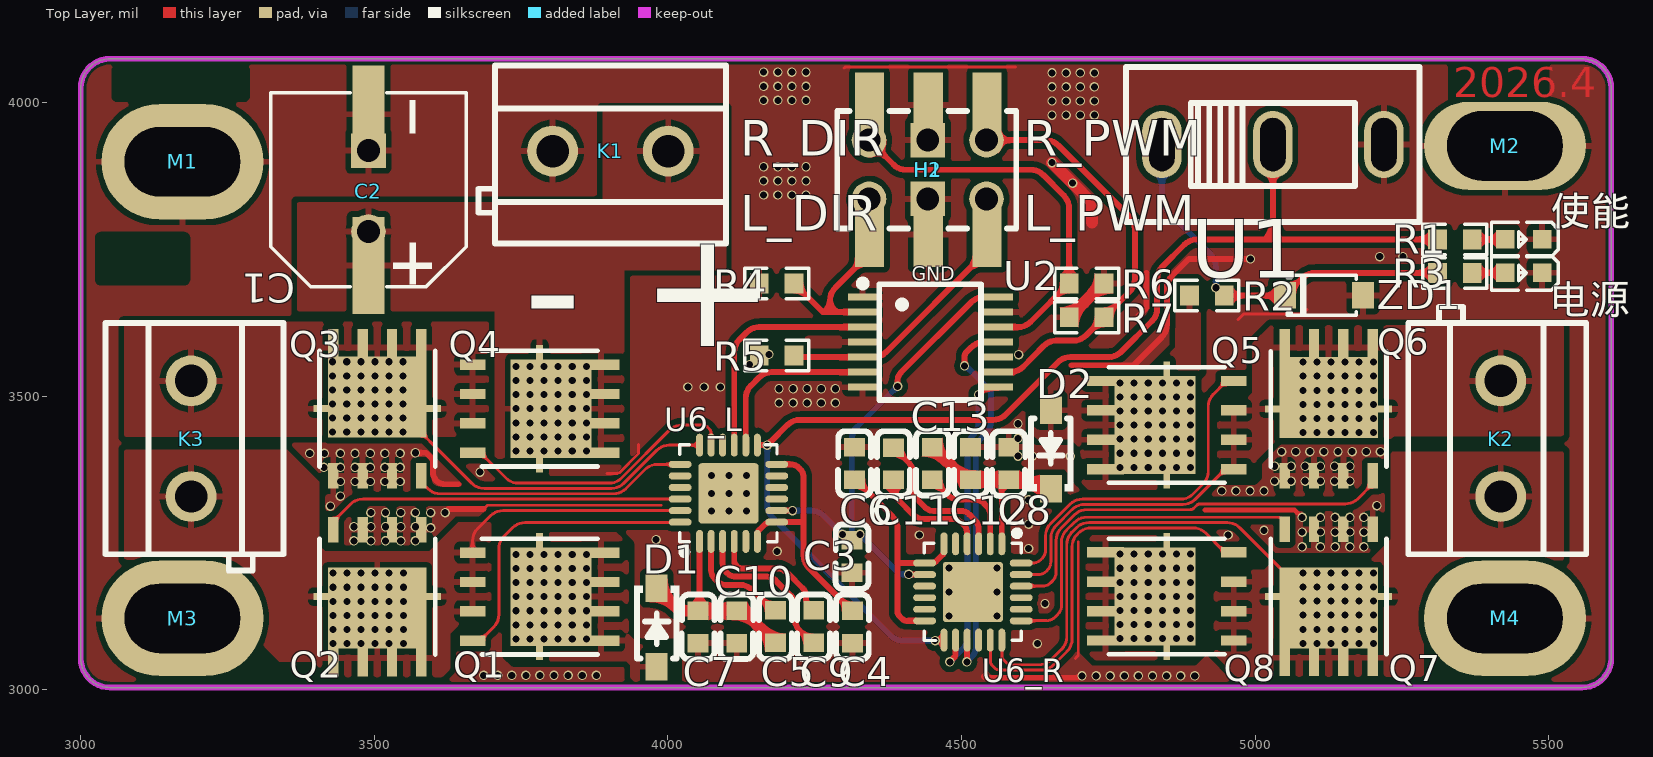
[diagram p0: Top Layer view]
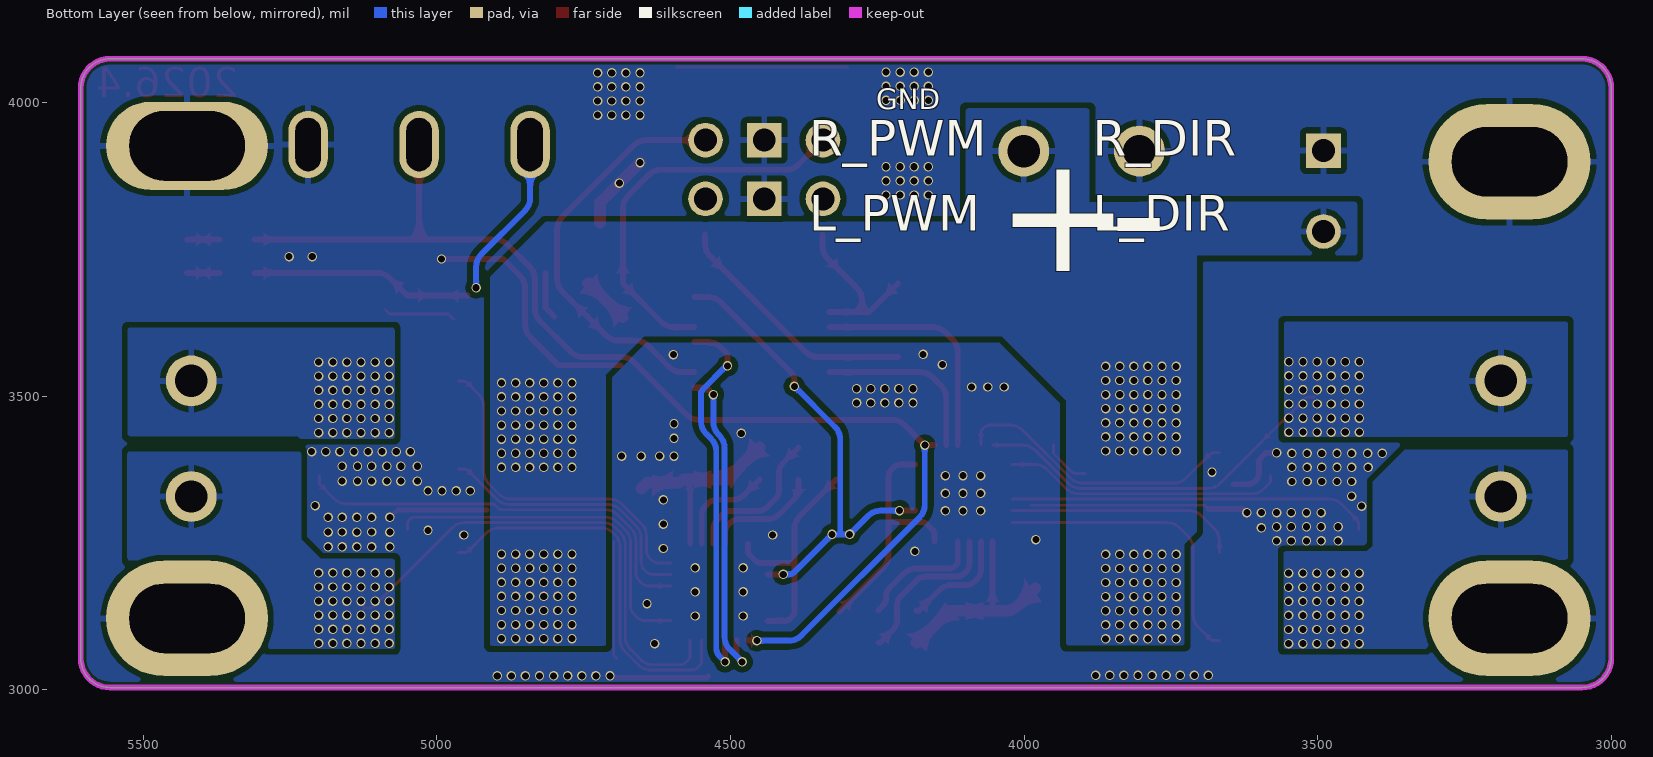
[diagram p1: Bottom Layer view, seen from below]
# Altium PCB MISC62357.pcbdoc (part 1 of 2)
Units mil, origin at the board's own origin, x right, y up, seen from the top; angles counter-clockwise.
Board outline 2606.3 x 1070.87 mil, 2 copper layers (Top Layer, Bottom Layer), stack 62.206 mil thick; 46 components, 37 nets, 219 pads, 514 vias.

## Layer stack, top to bottom
Top Solder Mask Layer: solder mask 0.394, Dk 3.3
Top Layer: signal copper 1.379
Dielectric1: surface 59.449, FR4, Dk 4.5
Bottom Layer: signal copper 1.378
Bottom Solder Mask Layer: solder mask 0.394, Dk 3.3

## Board outline
3050,4074.6 ccw(c3050,4024.6) 3000,4024.6 3000,3053.73 ccw(c3050,3053.73) 3050,3003.73 5556.3,3003.73 ccw(c5556.3,3053.73) 5606.3,3053.73 5606.3,4024.6 ccw(c5556.3,4024.6) 5556.3,4074.6

## Design rules (kind name [scope] priority, off if disabled: settings)
BoardOutlineClearance copperThickness2oz_1 [All] p2 off: genericclearance=8 ignorepadtopadclearanceinfootprint=FALSE except(0: Arc-SplitContinuation Track-SplitContinuation SMDPad-SplitContinuation THPad-SplitContinuation Via-SplitContinuation Fill-SplitContinuation Region-SplitContinuation Poly-SplitContinuation Text-SplitContinuation Hole-SplitContinuation; 6: Arc-CutoutEdge Track-CutoutEdge SMDPad-CutoutEdge THPad-CutoutEdge Via-CutoutEdge Text-CutoutEdge; 6.9: Hole-OutlineEdge Hole-CutoutEdge; 10: Poly-OutlineEdge Poly-CutoutEdge; 11.8: Arc-OutlineEdge Track-OutlineEdge SMDPad-OutlineEdge THPad-OutlineEdge Via-OutlineEdge Fill-OutlineEdge Region-OutlineEdge Text-OutlineEdge Fill-CutoutEdge Region-CutoutEdge)
BoardOutlineClearance Plane_innerPlane_1 [All] p4 off: genericclearance=4 ignorepadtopadclearanceinfootprint=FALSE except(0: Arc-SplitContinuation Track-SplitContinuation SMDPad-SplitContinuation THPad-SplitContinuation Via-SplitContinuation Fill-SplitContinuation Region-SplitContinuation Poly-SplitContinuation Text-SplitContinuation Hole-SplitContinuation; 6: Arc-CutoutEdge Track-CutoutEdge SMDPad-CutoutEdge THPad-CutoutEdge Via-CutoutEdge Text-CutoutEdge; 6.9: Hole-OutlineEdge Hole-CutoutEdge; 10: Poly-OutlineEdge Poly-CutoutEdge; 11.8: Arc-OutlineEdge Track-OutlineEdge SMDPad-OutlineEdge THPad-OutlineEdge Via-OutlineEdge Fill-OutlineEdge Region-OutlineEdge Text-OutlineEdge Fill-CutoutEdge Region-CutoutEdge)
BoardOutlineClearance Copper_copperRegion_1 [All] p6 off: genericclearance=4 ignorepadtopadclearanceinfootprint=FALSE except(0: Arc-SplitContinuation Track-SplitContinuation SMDPad-SplitContinuation THPad-SplitContinuation Via-SplitContinuation Fill-SplitContinuation Region-SplitContinuation Poly-SplitContinuation Text-SplitContinuation Hole-SplitContinuation; 6: Arc-CutoutEdge Track-CutoutEdge SMDPad-CutoutEdge THPad-CutoutEdge Via-CutoutEdge Text-CutoutEdge; 6.9: Hole-OutlineEdge Hole-CutoutEdge; 10: Poly-OutlineEdge Poly-CutoutEdge; 11.8: Arc-OutlineEdge Track-OutlineEdge SMDPad-OutlineEdge THPad-OutlineEdge Via-OutlineEdge Fill-OutlineEdge Region-OutlineEdge Text-OutlineEdge Fill-CutoutEdge Region-CutoutEdge)
BoardOutlineClearance Copper_直连_1 [All] p8 off: genericclearance=4 ignorepadtopadclearanceinfootprint=FALSE except(0: Arc-SplitContinuation Track-SplitContinuation SMDPad-SplitContinuation THPad-SplitContinuation Via-SplitContinuation Fill-SplitContinuation Region-SplitContinuation Poly-SplitContinuation Text-SplitContinuation Hole-SplitContinuation; 6: Arc-CutoutEdge Track-CutoutEdge SMDPad-CutoutEdge THPad-CutoutEdge Via-CutoutEdge Text-CutoutEdge; 6.9: Hole-OutlineEdge Hole-CutoutEdge; 10: Poly-OutlineEdge Poly-CutoutEdge; 11.8: Arc-OutlineEdge Track-OutlineEdge SMDPad-OutlineEdge THPad-OutlineEdge Via-OutlineEdge Fill-OutlineEdge Region-OutlineEdge Text-OutlineEdge Fill-CutoutEdge Region-CutoutEdge)
BoardOutlineClearance Copper_18_1 [All] p10 off: genericclearance=4 ignorepadtopadclearanceinfootprint=FALSE except(0: Arc-SplitContinuation Track-SplitContinuation SMDPad-SplitContinuation THPad-SplitContinuation Via-SplitContinuation Fill-SplitContinuation Region-SplitContinuation Poly-SplitContinuation Text-SplitContinuation Hole-SplitContinuation; 6: Arc-CutoutEdge Track-CutoutEdge SMDPad-CutoutEdge THPad-CutoutEdge Via-CutoutEdge Text-CutoutEdge; 6.9: Hole-OutlineEdge Hole-CutoutEdge; 10: Poly-OutlineEdge Poly-CutoutEdge; 11.8: Arc-OutlineEdge Track-OutlineEdge SMDPad-OutlineEdge THPad-OutlineEdge Via-OutlineEdge Fill-OutlineEdge Region-OutlineEdge Text-OutlineEdge Fill-CutoutEdge Region-CutoutEdge)
BoardOutlineClearance Copper_18_copperThickness1oz_1 [All] p12 off: genericclearance=4 ignorepadtopadclearanceinfootprint=FALSE except(0: Arc-SplitContinuation Track-SplitContinuation SMDPad-SplitContinuation THPad-SplitContinuation Via-SplitContinuation Fill-SplitContinuation Region-SplitContinuation Poly-SplitContinuation Text-SplitContinuation Hole-SplitContinuation; 6: Arc-CutoutEdge Track-CutoutEdge SMDPad-CutoutEdge THPad-CutoutEdge Via-CutoutEdge Text-CutoutEdge; 6.9: Hole-OutlineEdge Hole-CutoutEdge; 10: Poly-OutlineEdge Poly-CutoutEdge; 11.8: Arc-OutlineEdge Track-OutlineEdge SMDPad-OutlineEdge THPad-OutlineEdge Via-OutlineEdge Fill-OutlineEdge Region-OutlineEdge Text-OutlineEdge Fill-CutoutEdge Region-CutoutEdge)
BoardOutlineClearance Copper_18_Copper_copperRegion_1 [All] p14 off: genericclearance=4 ignorepadtopadclearanceinfootprint=FALSE except(0: Arc-SplitContinuation Track-SplitContinuation SMDPad-SplitContinuation THPad-SplitContinuation Via-SplitContinuation Fill-SplitContinuation Region-SplitContinuation Poly-SplitContinuation Text-SplitContinuation Hole-SplitContinuation; 6: Arc-CutoutEdge Track-CutoutEdge SMDPad-CutoutEdge THPad-CutoutEdge Via-CutoutEdge Text-CutoutEdge; 6.9: Hole-OutlineEdge Hole-CutoutEdge; 10: Poly-OutlineEdge Poly-CutoutEdge; 11.8: Arc-OutlineEdge Track-OutlineEdge SMDPad-OutlineEdge THPad-OutlineEdge Via-OutlineEdge Fill-OutlineEdge Region-OutlineEdge Text-OutlineEdge Fill-CutoutEdge Region-CutoutEdge)
BoardOutlineClearance Copper_copperRegion_Copper_18_1 [All] p16 off: genericclearance=4 ignorepadtopadclearanceinfootprint=FALSE except(0: Arc-SplitContinuation Track-SplitContinuation SMDPad-SplitContinuation THPad-SplitContinuation Via-SplitContinuation Fill-SplitContinuation Region-SplitContinuation Poly-SplitContinuation Text-SplitContinuation Hole-SplitContinuation; 6: Arc-CutoutEdge Track-CutoutEdge SMDPad-CutoutEdge THPad-CutoutEdge Via-CutoutEdge Text-CutoutEdge; 6.9: Hole-OutlineEdge Hole-CutoutEdge; 10: Poly-OutlineEdge Poly-CutoutEdge; 11.8: Arc-OutlineEdge Track-OutlineEdge SMDPad-OutlineEdge THPad-OutlineEdge Via-OutlineEdge Fill-OutlineEdge Region-OutlineEdge Text-OutlineEdge Fill-CutoutEdge Region-CutoutEdge)
BoardOutlineClearance Copper_copperRegion_Copper_copperRegion_1 [All] p18 off: genericclearance=4 ignorepadtopadclearanceinfootprint=FALSE except(0: Arc-SplitContinuation Track-SplitContinuation SMDPad-SplitContinuation THPad-SplitContinuation Via-SplitContinuation Fill-SplitContinuation Region-SplitContinuation Poly-SplitContinuation Text-SplitContinuation Hole-SplitContinuation; 6: Arc-CutoutEdge Track-CutoutEdge SMDPad-CutoutEdge THPad-CutoutEdge Via-CutoutEdge Text-CutoutEdge; 6.9: Hole-OutlineEdge Hole-CutoutEdge; 10: Poly-OutlineEdge Poly-CutoutEdge; 11.8: Arc-OutlineEdge Track-OutlineEdge SMDPad-OutlineEdge THPad-OutlineEdge Via-OutlineEdge Fill-OutlineEdge Region-OutlineEdge Text-OutlineEdge Fill-CutoutEdge Region-CutoutEdge)
BoardOutlineClearance copperThickness1oz_1 [All] p20: genericclearance=4 ignorepadtopadclearanceinfootprint=FALSE except(0: Arc-SplitContinuation Track-SplitContinuation SMDPad-SplitContinuation THPad-SplitContinuation Via-SplitContinuation Fill-SplitContinuation Region-SplitContinuation Poly-SplitContinuation Text-SplitContinuation Hole-SplitContinuation; 6: Arc-CutoutEdge Track-CutoutEdge SMDPad-CutoutEdge THPad-CutoutEdge Via-CutoutEdge Text-CutoutEdge; 6.9: Hole-OutlineEdge Hole-CutoutEdge; 10: Poly-OutlineEdge Poly-CutoutEdge; 11.8: Arc-OutlineEdge Track-OutlineEdge SMDPad-OutlineEdge THPad-OutlineEdge Via-OutlineEdge Fill-OutlineEdge Region-OutlineEdge Text-OutlineEdge Fill-CutoutEdge Region-CutoutEdge)
Clearance copperThickness2oz [All] p1 off: gap=8 ignorepadtopadclearanceinfootprint=FALSE except(6: SMDPad-Track SMDPad-SMDPad THPad-Track SMDPad-THPad THPad-THPad Track-Via SMDPad-Via THPad-Via Via-Via Fill-SMDPad Region-SMDPad Fill-THPad Region-THPad Fill-Via Region-Via Arc-Track Arc-SMDPad Arc-THPad Arc-Via Fill-Arc Region-Arc Arc-Arc Text-Track SMDPad-Text Text-THPad Text-Via Fill-Text Region-Text Arc-Text Text-Text; 6.9: Hole-Track Hole-SMDPad Hole-THPad Hole-Via Fill-Hole Region-Hole Hole-Arc Hole-Text; 10: Poly-Track Poly-SMDPad Poly-THPad Poly-Via Poly-Fill Poly-Region Poly-Poly Poly-Arc Poly-Text Poly-Hole; 11.8: Fill-Track Region-Track; 20: Fill-Fill Fill-Region Region-Region)
Clearance Plane_innerPlane [All] p3 off: gap=4 ignorepadtopadclearanceinfootprint=FALSE except(6: SMDPad-Track SMDPad-SMDPad THPad-Track SMDPad-THPad THPad-THPad Track-Via SMDPad-Via THPad-Via Via-Via Fill-SMDPad Region-SMDPad Fill-THPad Region-THPad Fill-Via Region-Via Arc-Track Arc-SMDPad Arc-THPad Arc-Via Fill-Arc Region-Arc Arc-Arc Text-Track SMDPad-Text Text-THPad Text-Via Fill-Text Region-Text Arc-Text Text-Text; 6.9: Hole-Track Hole-SMDPad Hole-THPad Hole-Via Fill-Hole Region-Hole Hole-Arc Hole-Text; 10: Poly-Track Poly-SMDPad Poly-THPad Poly-Via Poly-Fill Poly-Region Poly-Poly Poly-Arc Poly-Text Poly-Hole; 11.8: Fill-Track Region-Track; 12: Fill-Fill Fill-Region Region-Region)
Clearance Copper_copperRegion [All] p5 off: gap=4 ignorepadtopadclearanceinfootprint=FALSE except(6: SMDPad-Track SMDPad-SMDPad THPad-Track SMDPad-THPad THPad-THPad Track-Via SMDPad-Via THPad-Via Via-Via Fill-SMDPad Region-SMDPad Fill-THPad Region-THPad Fill-Via Region-Via Arc-Track Arc-SMDPad Arc-THPad Arc-Via Fill-Arc Region-Arc Arc-Arc Text-Track SMDPad-Text Text-THPad Text-Via Fill-Text Region-Text Arc-Text Text-Text; 6.9: Hole-Track Hole-SMDPad Hole-THPad Hole-Via Fill-Hole Region-Hole Hole-Arc Hole-Text; 10: Poly-Track Poly-SMDPad Poly-THPad Poly-Via Poly-Fill Poly-Region Poly-Poly Poly-Arc Poly-Text Poly-Hole; 11.8: Fill-Track Region-Track; 12: Fill-Fill Fill-Region Region-Region)
Clearance Copper_直连 [All] p7 off: gap=4 ignorepadtopadclearanceinfootprint=FALSE except(6: SMDPad-Track SMDPad-SMDPad THPad-Track SMDPad-THPad THPad-THPad Track-Via SMDPad-Via THPad-Via Via-Via Fill-SMDPad Region-SMDPad Fill-THPad Region-THPad Fill-Via Region-Via Arc-Track Arc-SMDPad Arc-THPad Arc-Via Fill-Arc Region-Arc Arc-Arc Text-Track SMDPad-Text Text-THPad Text-Via Fill-Text Region-Text Arc-Text Text-Text; 6.9: Hole-Track Hole-SMDPad Hole-THPad Hole-Via Fill-Hole Region-Hole Hole-Arc Hole-Text; 10: Poly-Track Poly-SMDPad Poly-THPad Poly-Via Poly-Fill Poly-Region Poly-Poly Poly-Arc Poly-Text Poly-Hole; 11.8: Fill-Track Region-Track; 12: Fill-Fill Fill-Region Region-Region)
Clearance Copper_18 [All] p9 off: gap=4 ignorepadtopadclearanceinfootprint=FALSE except(6: SMDPad-Track SMDPad-SMDPad THPad-Track SMDPad-THPad THPad-THPad Track-Via SMDPad-Via THPad-Via Via-Via Fill-SMDPad Region-SMDPad Fill-THPad Region-THPad Fill-Via Region-Via Arc-Track Arc-SMDPad Arc-THPad Arc-Via Fill-Arc Region-Arc Arc-Arc Text-Track SMDPad-Text Text-THPad Text-Via Fill-Text Region-Text Arc-Text Text-Text; 6.9: Hole-Track Hole-SMDPad Hole-THPad Hole-Via Fill-Hole Region-Hole Hole-Arc Hole-Text; 10: Poly-Track Poly-SMDPad Poly-THPad Poly-Via Poly-Fill Poly-Region Poly-Poly Poly-Arc Poly-Text Poly-Hole; 11.8: Fill-Track Region-Track; 12: Fill-Fill Fill-Region Region-Region)
Clearance Copper_18_copperThickness1oz [All] p11 off: gap=4 ignorepadtopadclearanceinfootprint=FALSE except(6: SMDPad-Track SMDPad-SMDPad THPad-Track SMDPad-THPad THPad-THPad Track-Via SMDPad-Via THPad-Via Via-Via Fill-SMDPad Region-SMDPad Fill-THPad Region-THPad Fill-Via Region-Via Arc-Track Arc-SMDPad Arc-THPad Arc-Via Fill-Arc Region-Arc Arc-Arc Text-Track SMDPad-Text Text-THPad Text-Via Fill-Text Region-Text Arc-Text Text-Text; 6.9: Hole-Track Hole-SMDPad Hole-THPad Hole-Via Fill-Hole Region-Hole Hole-Arc Hole-Text; 10: Poly-Track Poly-SMDPad Poly-THPad Poly-Via Poly-Fill Poly-Region Poly-Poly Poly-Arc Poly-Text Poly-Hole; 11.8: Fill-Track Region-Track; 12: Fill-Fill Fill-Region Region-Region)
Clearance Copper_18_Copper_copperRegion [All] p13 off: gap=4 ignorepadtopadclearanceinfootprint=FALSE except(6: SMDPad-Track SMDPad-SMDPad THPad-Track SMDPad-THPad THPad-THPad Track-Via SMDPad-Via THPad-Via Via-Via Fill-SMDPad Region-SMDPad Fill-THPad Region-THPad Fill-Via Region-Via Arc-Track Arc-SMDPad Arc-THPad Arc-Via Fill-Arc Region-Arc Arc-Arc Text-Track SMDPad-Text Text-THPad Text-Via Fill-Text Region-Text Arc-Text Text-Text; 6.9: Hole-Track Hole-SMDPad Hole-THPad Hole-Via Fill-Hole Region-Hole Hole-Arc Hole-Text; 10: Poly-Track Poly-SMDPad Poly-THPad Poly-Via Poly-Fill Poly-Region Poly-Poly Poly-Arc Poly-Text Poly-Hole; 11.8: Fill-Track Region-Track; 12: Fill-Fill Fill-Region Region-Region)
Clearance Copper_copperRegion_Copper_18 [All] p15 off: gap=4 ignorepadtopadclearanceinfootprint=FALSE except(6: SMDPad-Track SMDPad-SMDPad THPad-Track SMDPad-THPad THPad-THPad Track-Via SMDPad-Via THPad-Via Via-Via Fill-SMDPad Region-SMDPad Fill-THPad Region-THPad Fill-Via Region-Via Arc-Track Arc-SMDPad Arc-THPad Arc-Via Fill-Arc Region-Arc Arc-Arc Text-Track SMDPad-Text Text-THPad Text-Via Fill-Text Region-Text Arc-Text Text-Text; 6.9: Hole-Track Hole-SMDPad Hole-THPad Hole-Via Fill-Hole Region-Hole Hole-Arc Hole-Text; 10: Poly-Track Poly-SMDPad Poly-THPad Poly-Via Poly-Fill Poly-Region Poly-Poly Poly-Arc Poly-Text Poly-Hole; 11.8: Fill-Track Region-Track; 12: Fill-Fill Fill-Region Region-Region)
Clearance Copper_copperRegion_Copper_copperRegion [All] p17 off: gap=4 ignorepadtopadclearanceinfootprint=FALSE except(6: SMDPad-Track SMDPad-SMDPad THPad-Track SMDPad-THPad THPad-THPad Track-Via SMDPad-Via THPad-Via Via-Via Fill-SMDPad Region-SMDPad Fill-THPad Region-THPad Fill-Via Region-Via Arc-Track Arc-SMDPad Arc-THPad Arc-Via Fill-Arc Region-Arc Arc-Arc Text-Track SMDPad-Text Text-THPad Text-Via Fill-Text Region-Text Arc-Text Text-Text; 6.9: Hole-Track Hole-SMDPad Hole-THPad Hole-Via Fill-Hole Region-Hole Hole-Arc Hole-Text; 10: Poly-Track Poly-SMDPad Poly-THPad Poly-Via Poly-Fill Poly-Region Poly-Poly Poly-Arc Poly-Text Poly-Hole; 11.8: Fill-Track Region-Track; 12: Fill-Fill Fill-Region Region-Region)
Clearance copperThickness1oz [All] p19: gap=4 ignorepadtopadclearanceinfootprint=FALSE except(6: SMDPad-Track SMDPad-SMDPad THPad-Track SMDPad-THPad THPad-THPad Track-Via SMDPad-Via THPad-Via Via-Via Fill-SMDPad Region-SMDPad Fill-THPad Region-THPad Fill-Via Region-Via Arc-Track Arc-SMDPad Arc-THPad Arc-Via Fill-Arc Region-Arc Arc-Arc Text-Track SMDPad-Text Text-THPad Text-Via Fill-Text Region-Text Arc-Text Text-Text; 6.9: Hole-Track Hole-SMDPad Hole-THPad Hole-Via Fill-Hole Region-Hole Hole-Arc Hole-Text; 10: Poly-Track Poly-SMDPad Poly-THPad Poly-Via Poly-Fill Poly-Region Poly-Poly Poly-Arc Poly-Text Poly-Hole; 11.8: Fill-Track Region-Track; 12: Fill-Fill Fill-Region Region-Region)
DiffPairsRouting differentialPair [All] p1: maxlimit=6 minlimit=6 mostfreqgap=6 toplayer_minwidth=5 toplayer_prefwidth=10 toplayer_maxwidth=100 toplayer_mingap=6 toplayer_prefgap=6 toplayer_maxgap=6 bottomlayer_minwidth=5 bottomlayer_prefwidth=10 bottomlayer_maxwidth=100 bottomlayer_mingap=6 bottomlayer_prefgap=6 bottomlayer_maxgap=6 maxuncoupledlength=10
HoleToHoleClearance otherClearance [All] p1: gap=11.8 allowstackedmicrovias=TRUE
Length netLength [All] p1: minlimit=0 maxlimit=0
PasteMaskExpansion pasteMaskExpansion [All] p1: expansion=0
PlaneConnect innerPlane [All] p1: planeconnectstyle=Relief reliefexpansion=20 reliefentries=4 reliefconductorwidth=10 reliefairgap=10
PolygonConnect 直连 [All] p1 off: connectstyle=Direct reliefconductorwidth=10 reliefentries=4 polygonreliefangle="90 Angle" airgapwidth=10 via.connectstyle=Relief via.reliefconductorwidth=10 via.reliefentries=4 via.polygonreliefangle="90 Angle" via.airgapwidth=10
PolygonConnect 18 [All] p2 off: connectstyle=Relief reliefconductorwidth=10 reliefentries=4 polygonreliefangle="90 Angle" airgapwidth=10 smdpad.connectstyle=Direct via.connectstyle=Relief via.reliefconductorwidth=10 via.reliefentries=4 via.polygonreliefangle="90 Angle" via.airgapwidth=10
PolygonConnect 18_copperThickness1oz [All] p3 off: connectstyle=Relief reliefconductorwidth=10 reliefentries=4 polygonreliefangle="90 Angle" airgapwidth=10 via.connectstyle=Relief via.reliefconductorwidth=10 via.reliefentries=4 via.polygonreliefangle="90 Angle" via.airgapwidth=10
PolygonConnect 18_Copper_copperRegion [All] p4 off: connectstyle=Relief reliefconductorwidth=10 reliefentries=4 polygonreliefangle="90 Angle" airgapwidth=10 via.connectstyle=Relief via.reliefconductorwidth=10 via.reliefentries=4 via.polygonreliefangle="90 Angle" via.airgapwidth=10
PolygonConnect copperRegion_Copper_18 [All] p5 off: connectstyle=Relief reliefconductorwidth=10 reliefentries=4 polygonreliefangle="90 Angle" airgapwidth=10 via.connectstyle=Relief via.reliefconductorwidth=10 via.reliefentries=4 via.polygonreliefangle="90 Angle" via.airgapwidth=10
PolygonConnect copperRegion_Copper_copperRegion [All] p6 off: connectstyle=Relief reliefconductorwidth=10 reliefentries=4 polygonreliefangle="90 Angle" airgapwidth=10 via.connectstyle=Relief via.reliefconductorwidth=10 via.reliefentries=4 via.polygonreliefangle="90 Angle" via.airgapwidth=10
PolygonConnect copperRegion [All] p7: connectstyle=Relief reliefconductorwidth=10 reliefentries=4 polygonreliefangle="90 Angle" airgapwidth=10 smdpad.connectstyle=Direct via.connectstyle=Relief via.reliefconductorwidth=10 via.reliefentries=4 via.polygonreliefangle="90 Angle" via.airgapwidth=10
RoutingVias viaSize [All] p1: holewidth=12 width=24 viastyle="Through Hole" minholewidth=11.8 minwidth=15.7 maxholewidth=248 maxwidth=393.7
SolderMaskExpansion solderMaskExpansion [IsVia] p1: expansion=-1000 istentingtop=TRUE
SolderMaskExpansion solderMaskExpansion [All] p2: expansion=2 istentingtop=FALSE
Width copperThickness2oz_2 [All] p1 off: maxlimit=100 minlimit=8 preferedwidth=10
Width copperThickness1oz_2 [All] p2: maxlimit=100 minlimit=5 preferedwidth=10

## Components (designator, comment, footprint, x,y, rotation, side; value= is the part's Value field where it differs from the comment)
C1 "220uF" CAP-SMD_BD8.0-L8.3-W8.3-FD 3490,3851.4 r90 top
C2 "220uF" CAP-TH_BD8.0-P3.50-D0.6-FD 3490,3849.19 r90 top
C3 "1UF" C0603 4313.61,3226.94 r90 top
C4 "1UF" C0603 4314.03,3106.95 r270 top
C5 "1UF" C0603 4183,3107.56 r90 top
C6 "1UF" C0603 4317.88,3385.6 r90 top
C7 "10UF" C0603 4051.33,3106.95 r270 top
C8 "10UF" C0603 4580.36,3385.6 r90 top
C9 "100nF" C0603 4248.12,3107.56 r90 top
C10 "100nF" C0603 4117.14,3106.95 r270 top
C11 "100nF" C0603 4383.79,3384.99 r270 top
C12 "100nF" C0603 4515.24,3385.6 r90 top
C13 "1UF" C0603 4450.12,3385.6 r270 top
D1 "1N5819W" SOD-123_L2.7-W1.6-LS3.7-RD-1 3980.81,3106.05 r270 top
D2 "1N5819W" SOD-123_L2.7-W1.6-LS3.7-RD-1 4651.88,3409.05 r90 top
H1 "SMD" HDR-SMD_6P-P2.54-V-M-R2-C5-S7.4 4443.16,3885.68 r0 top locked
H2 "" HDR-TH_6P-P2.54-V-R2-C3-S2.54_A2541WV-2X3P 4442.39,3885.88 r0 top locked
K1 "KF301-5.0-2P" CONN-TH_P5.00_KF301-5.0-2P 3902,3917.23 r180 top
K2 "KF301-5.0-2P" CONN-TH_P5.00_KF301-5.0-2P 5418,3427.56 r90 top
K3 "KF301-5.0-2P" CONN-TH_P5.00_KF301-5.0-2P 3188,3427.56 r270 top
M1 "" M4螺丝#1 3173.23,3899.12 r0 top
M2 "" M4螺丝#2 5425.2,3926.25 r0 top
M3 "" M4螺丝#1 3173.23,3121.56 r0 top
M4 "" M4螺丝#1 5425.2,3121.56 r0 top
Q1 "TPH1R403NL" DFN5x6 3781.49,3158.6 r270 top
Q2 "TPH1R403NL" DFN5x6 3505,3158.6 r180 top
Q3 "TPH1R403NL" DFN5x6 3505,3478.6 r0 top
Q4 "TPH1R403NL" DFN5x6 3781.49,3478.6 r270 top
Q5 "TPH1R403NL" DFN5x6 4849.3,3450.76 r90 top
Q6 "TPH1R403NL" DFN5x6 5125,3478.32 r0 top
Q7 "TPH1R403NL" DFN5x6 5125,3158.96 r180 top
Q8 "TPH1R403NL" DFN5x6 4849.3,3158.96 r90 top
R1 "2.2K" R0603 5340,3766.89 r180 top
R2 "2.2K" R0603 4917.65,3671.08 r180 top
R3 "2.2K" R0603 5340,3709.87 r180 top
R4 "10K" R0603 4185,3692.07 r180 top
R5 "10K" R0603 4185,3569.37 r180 top
R6 "10K" R0603 4712.79,3692.07 r180 top
R7 "10K" R0603 4712.79,3634.37 r0 top
U1 "SS12D10G5" SW-TH_SHOU-HAN_SS12D10G4 5030,3928.47 r0 top
U2 "SN74HC125PWR" TSSOP-14_L5.0-W4.4-P0.65-LS6.5-BL 4446.48,3592.03 r270 top
U6_L "DRV8701ERGET" VQFN-24_L4.0-W4.0-P0.50-BL-EP2.5 4103,3334.6 r0 top
U6_R "DRV8701ERGET" VQFN-24_L4.0-W4.0-P0.50-BL-EP2.5 4519.24,3166.6 r180 top
ZD1 "BZT52C3V6" SOD-123_L2.8-W1.8-LS3.7-RD 5117,3671.48 r0 top
使能 "" LED_0603 5455,3766.79 r180 top
电源 "" LED_0603 5455,3709.77 r180 top

## Footprints (in the part's own frame and the unit in brackets; to place one, negate y for a bottom-side part, rotate by r counter-clockwise, add the part's x,y. Pads: shape width x height; smd on the part's side, far side on the other; paste and mask are expansions set on the pad)
C0603 [mm]
  rect 0.8x0.9 smd: 1(-0.7,0) 2(0.7,0)
  silkscreen extent -1.41,-0.71 1.39,0.72
CAP-SMD_BD8.0-L8.3-W8.3-FD [mm]
  rect 4.2x1.4 smd: 1(-3.267,0) 2(3.267,0)
  silkscreen extent -4.2,-4.23 4.2,4.23
CAP-TH_BD8.0-P3.50-D0.6-FD [mil]
  round 59 hole 39: 1(-68.9,0)
  rect 59x59 hole 39: 2(68.9,0)
CONN-TH_P5.00_KF301-5.0-2P [mm]
  round 2.2 hole 1.4: 1(-2.5,0) 2(2.5,0)
  silkscreen extent -5,-3.7 5.71,4
DFN5x6 [mm]
  rect 0.45x1.6 smd: 1(-1.905,2.65) 1(-0.635,2.65) 1(0.635,2.65) 1(1.905,2.65)
  rect 5.5x0.3 smd: 1(0,0)
  rect 4.25x3.5 smd: 1(0,0.5)
  rect 0.45x1.1 smd: 2(1.905,-2.9) 3(-1.905,-2.9) 3(-0.635,-2.9) 3(0.635,-2.9)
  silkscreen extent -2.5,-2.5 2.5,2.5
HDR-SMD_6P-P2.54-V-M-R2-C5-S7.4 [mm]
  rect 1.27x2.8 smd: 1(-2.54,-2.8) 2(-2.54,2.8) 3(0,-2.8) 4(0,2.8) 5(2.54,-2.8) 6(2.54,2.8)
  silkscreen extent -3.94,-2.54 3.81,2.54
HDR-TH_6P-P2.54-V-R2-C3-S2.54_A2541WV-2X3P [mil]
  round 59 hole 39: 1(-100,-50) 2(-100,50) 5(100,-50) 6(100,50)
  rect 59x59 hole 39: 3(0,-50) 4(0,50)
LED_0603 [mil]
  rect 31.5x31.5 smd paste+0 mask+2: 1(-33.5,-0.4) 2(29.5,-0.2)
  silkscreen extent -61,-30 53,30
M4螺丝#1 [mm]
  oval 7x5 hole 3 slot 5 at 0 deg paste+0 mask+0.127: 1(0,0)
M4螺丝#2 [mm]
  oval 7x3.81 hole 3 slot 5 at 0 deg paste+0 mask+0.127: 1(0,0)
R0603 [mil]
  rect 31.75x34.02 smd paste-3937.01 mask+2: 1(-29.66,0) 2(29.66,0)
  silkscreen extent -55,-26 55,26
SOD-123_L2.7-W1.6-LS3.7-RD-1 [mm]
  rect 1.2x0.95 smd: 1(-1.7,0) 2(1.7,0)
  silkscreen extent -1.81,-0.98 1.35,0.98
SOD-123_L2.8-W1.8-LS3.7-RD [mm]
  rect 0.95x1.15 smd: 1(-1.692,0) 2(1.692,0)
  silkscreen extent -1.58,-0.87 1.41,0.87
SW-TH_SHOU-HAN_SS12D10G4 [mm]
  oval 1.7x2.9 hole 1.1 slot 2.3 at 90 deg paste+0 mask+0.05: 1(-4.8,0) 2(0,0) 3(4.8,0)
  silkscreen extent -6.35,-3.35 6.35,3.35
TSSOP-14_L5.0-W4.4-P0.65-LS6.5-BL [mil]
  rect 12x50 smd paste+0 mask+1.97: 1(-76.77,-115.16) 2(-51.18,-115.16) 3(-25.59,-115.16) 4(0,-115.16) 5(25.59,-115.16) 6(51.18,-115.16) 7(76.77,-115.16) 8(76.77,116.16) 9(51.18,116.16) 10(25.59,116.16) 11(0,116.16) 12(-25.59,116.16) 13(-51.18,116.16) 14(-76.77,116.16)
  silkscreen extent -106,-121 98,87
VQFN-24_L4.0-W4.0-P0.50-BL-EP2.5 [mil]
  rrect100% 11.81x39 smd paste-3937 mask+2: 1(-49.21,-81.95) 2(-29.53,-81.95) 3(-9.84,-81.95) 4(9.84,-81.95) 5(29.53,-81.95) 6(49.21,-81.95) 13(49.21,81.96) 14(29.53,81.96) 15(9.84,81.96) 16(-9.84,81.96) 17(-29.53,81.96) 18(-49.21,81.96)
  rrect100% 39x11.81 smd paste-3937 mask+2: 7(82.2,-49.21) 8(82.2,-29.52) 9(82.2,-9.84) 10(82.2,9.84) 11(82.2,29.53) 12(82.2,49.21) 19(-82.2,49.21) 20(-82.2,29.53) 21(-82.2,9.84) 22(-82.2,-9.84) 23(-82.2,-29.52) 24(-82.2,-49.21)
  rrect10% 102.36x102.36 smd paste-3937 mask+2: 25(0.03,-0.03)
  silkscreen extent -83,-105 83,83

## Via types
v1: diameter 16, hole 12, Top Layer to Bottom Layer, 514 vias

## Nets (pads, with @x,y where several pads share a name; then routed paths per layer and width w, separated by ;. In a path a pad name is that pad's centre, name@x,y a point inside that pad or via, vN(x,y) a via of type N, cw(c..) or ccw(c..) an arc to the next point about the centre after c; other vN are vias at no path point)
3V6: R2.1 R3.2 U1.1 ZD1.1 | length 657.2
  Top Layer w10: R2.1@4947.31,3671.08 5049.98,3671.08 ZD1.1@5050.37,3671.48 5079.98,3701.09 cw(c5101.19,3679.87) 5101.19,3709.87 R3.2@5310.34,3709.87
  Bottom Layer w10: 4841.02,3837 U1.1@4841.02,3928.47 ; 4841.03,3837 ccw(c4871.02,3837) 4849.81,3815.79 4924.21,3741.39 cw(c4903,3720.17) 4933,3720.17 v1(4933,3684.6)
$1N440: R1.1 使能.2 | length 55.9
  Top Layer w10: R1.1@5369.66,3766.89 5425.4,3766.89 使能.2@5425.5,3766.99
$1N595: R3.1 电源.2 | length 55.9
  Top Layer w10: R3.1@5369.66,3709.87 5369.76,3709.97 电源.2@5425.5,3709.97
$1N3022: C9.1 U6_L.3 | length 274.9
  Top Layer w10: U6_L.3@4093.16,3252.65 4093.16,3214.73 ccw(c4113.16,3214.73) 4099.02,3200.58 4101.14,3198.46 ccw(c4115.28,3212.6) 4115.28,3192.6 4168.72,3192.6 cw(c4168.72,3172.6) 4182.86,3186.74 4210.14,3159.46 cw(c4196,3145.32) 4216,3145.32 4216,3121.47 ccw(c4246,3121.47) 4224.79,3100.26 4245.04,3080 C9.1@4248.12,3080
$1N3052: C9.2 U6_L.4 | length 213.4
  Top Layer w10: U6_L.4@4112.84,3252.65 4112.84,3219.35 ccw(c4122.84,3219.35) 4115.77,3212.27 4118.48,3209.56 ccw(c4125.55,3216.63) 4125.55,3206.63 4183.54,3206.63 cw(c4183.54,3176.63) 4204.76,3197.84 4229.14,3173.46 cw(c4215,3159.32) 4235,3159.32 4235,3156.53 ccw(c4255,3156.53) 4240.86,3142.38 C9.2@4248.12,3135.12
$1N3247: C5.2 U6_L.2 | length 188.9
  Top Layer w10: U6_L.2@4073.47,3252.65 4073.47,3203.42 ccw(c4093.47,3203.42) 4079.33,3189.27 4084.14,3184.46 ccw(c4098.28,3198.6) 4098.28,3178.6 4122.57,3178.6 cw(c4122.57,3148.6) 4143.79,3169.81 4178.48,3135.12 C5.2@4183,3135.12
$1N3253: C5.1 C7.1 C10.1 D1.1 U6_L.1 | length 358.7
  Top Layer w10: C7.1@4051.33,3134.51 4053.79,3136.97 U6_L.1@4053.79,3252.65
  Top Layer w20: D1.1@3980.81,3172.98 4010.49,3143.3 ccw(c4031.7,3164.51) 4031.7,3134.51 C7.1@4051.33,3134.51 C10.1@4117.14,3134.51 4124.35,3134.51 cw(c4124.35,3124.51) 4131.42,3131.58 4149.3,3113.7 4149.3,3112.75 4158.66,3103.39 4159.61,3103.39 C5.1@4183,3080
$1N4029: C11.1 U6_R.3 | length 256.8
  Top Layer w10: C11.1@4383.79,3412.55 4411.14,3385.19 cw(c4397,3371.05) 4417,3371.05 4417,3339.81 ccw(c4437,3339.81) 4422.86,3325.67 4438.07,3310.46 ccw(c4452.21,3324.6) 4452.21,3304.6 4498.72,3304.6 cw(c4498.72,3284.6) 4512.86,3298.74 4523.22,3288.38 cw(c4509.08,3274.24) 4529.08,3274.24 U6_R.3@4529.08,3248.55
$1N4031: C11.2 U6_R.4 | length 197
  Top Layer w10: C11.2@4383.79,3357.43 4383.79,3344.24 ccw(c4413.79,3344.24) 4392.58,3323.03 4416.21,3299.39 ccw(c4437.43,3320.6) 4437.43,3290.6 4485.72,3290.6 cw(c4485.72,3270.6) 4499.86,3284.74 4503.54,3281.06 cw(c4489.4,3266.92) 4509.4,3266.92 U6_R.4@4509.4,3248.55
$1N4034: C13.2 U6_R.2 | length 175.1
  Top Layer w10: C13.2@4450.12,3358.04 4475.77,3332.39 ccw(c4496.98,3353.6) 4496.98,3323.6 4523.72,3323.6 cw(c4523.72,3303.6) 4537.86,3317.74 4542.91,3312.69 cw(c4528.77,3298.55) 4548.77,3298.55 U6_R.2@4548.77,3248.55
$1N4036: C8.1 C12.1 C13.1 D2.1 U6_R.1 | length 335.5
  Top Layer w10: U6_R.1@4568.45,3248.55 4568.45,3337.84 cw(c4588.45,3337.84) 4574.31,3351.98 C8.1@4580.36,3358.04
  Top Layer w20: C13.1@4450.12,3413.16 4473.51,3389.77 4474.46,3389.77 4483.82,3380.4 4483.82,3379.45 4502.31,3360.96 ccw(c4509.38,3368.04) 4509.38,3358.04 C12.1@4515.24,3358.04 C8.1@4580.36,3358.04 ; C8.1@4586.96,3352.44 D2.1@4642.56,3352.44 ; D2.1@4642.56,3351.44 D2.1@4651.88,3342.12
AVDD_L: C4.1 U6_L.6 U6_L.7 U6_L.12 | length 420.9
  Top Layer w10: U6_L.6@4152.21,3252.65 4152.21,3264.71 cw(c4162.21,3264.71) 4155.14,3271.78 4165.82,3282.46 cw(c4172.89,3275.39) 4172.89,3285.39 U6_L.7@4185.2,3285.39 4229.01,3285.39 4230.98,3287.36 ; U6_L.12@4185.2,3383.81 4208.51,3383.81 cw(c4208.51,3363.81) 4222.65,3377.95 4225.13,3375.47 cw(c4210.98,3361.33) 4230.98,3361.33 4230.98,3287.36 ; C4.1@4314.03,3133.51 4239.77,3207.77 cw(c4260.98,3228.98) 4230.98,3228.98 4230.98,3287.36
AVDD_R: C6.1 U6_R.6 U6_R.7 U6_R.12 | length 410.4
  Top Layer w10: C6.1@4317.88,3358.04 4319.56,3358.04 4382.23,3295.37 cw(c4361.02,3274.16) 4391.02,3274.16 4391.02,3215.81 ; U6_R.12@4437.04,3117.39 4406.35,3117.39 cw(c4406.35,3127.39) 4399.28,3120.32 4393.94,3125.66 cw(c4401.02,3132.73) 4391.02,3132.73 4391.02,3215.81 ; U6_R.6@4470.03,3248.55 4470.03,3236.49 cw(c4460.03,3236.49) 4467.1,3229.42 4456.42,3218.74 cw(c4449.35,3225.81) 4449.35,3215.81 U6_R.7@4437.04,3215.81 4391.02,3215.81
D3V3: C3.2 U2.14 U6_L.8 U6_R.8 | length 819.5
  Top Layer w10: U6_L.8@4185.2,3305.08 v1(4212,3305.08) ; v1(4391,3516.6) 4391,3526.32 cw(c4411,3526.32) 4396.86,3540.46 4516.41,3660.01 cw(c4537.62,3638.8) 4537.62,3668.8 U2.14@4561.64,3668.8 ; v1(4410,3196.6) 4410.48,3196.12 U6_R.8@4437.04,3196.12
  Bottom Layer w10: v1(4212,3305.08) 4244.1,3305.08 cw(c4244.1,3275.08) 4265.31,3296.29 4294.07,3267.53 ccw(c4301.14,3274.6) 4301.14,3264.6 4313,3264.6 ; v1(4391,3516.6) 4321.79,3447.39 ccw(c4343,3426.17) 4313,3426.17 4313,3264.6 ; v1(4410,3196.6) 4399.14,3196.6 cw(c4399.14,3206.6) 4392.07,3199.53 4329.93,3261.67 ccw(c4322.86,3254.6) 4322.86,3264.6 4313,3264.6
  other v1: 4297,3264.6 4327,3264.6
GH1_L: Q4.2 U6_L.17 | length 491.9
  Top Layer w5: Q4.2@3667.31,3403.6 3676.86,3403.6 cw(c3676.86,3393.6) 3683.93,3400.67 3724.01,3360.59 ccw(c3745.22,3381.8) 3745.22,3351.8 3899.78,3351.8 ccw(c3899.78,3381.8) 3920.99,3360.59 4002.21,3441.81 cw(c4023.43,3420.6) 4023.43,3450.6 4059.86,3450.6 cw(c4059.86,3440.6) 4066.93,3447.67 4070.54,3444.06 cw(c4063.47,3436.99) 4073.47,3436.99 U6_L.17@4073.47,3416.56
GH1_R: Q8.2 U6_R.17 | length 675.5
  Top Layer w5: U6_R.17@4548.77,3084.64 4549,3084.41 4549,3048.74 ccw(c4559,3048.74) 4551.93,3041.67 4557.07,3036.53 ccw(c4564.14,3043.6) 4564.14,3033.6 4635.32,3033.6 ccw(c4635.32,3063.6) 4656.54,3042.39 4679.26,3065.11 ccw(c4658.05,3086.32) 4688.05,3086.32 4688.05,3243.29 cw(c4718.05,3243.29) 4696.83,3264.51 4699.26,3266.93 cw(c4720.47,3245.71) 4720.47,3275.71 4894.46,3275.71 cw(c4894.46,3245.71) 4915.67,3266.93 4945.71,3236.89 ccw(c4952.78,3243.96) 4952.78,3233.96 Q8.2@4963.47,3233.96
GH2_L: Q1.2 U6_L.24 | length 513
  Top Layer w5: Q1.2@3667.31,3083.6 3675.86,3083.6 ccw(c3675.86,3093.6) 3682.93,3086.53 3703.21,3106.81 ccw(c3682,3128.03) 3712,3128.03 3712,3240.17 cw(c3742,3240.17) 3720.79,3261.39 3735.21,3275.81 cw(c3756.43,3254.6) 3756.43,3284.6 4020.01,3284.6 U6_L.24@4020.8,3285.39
GH2_R: Q5.2 U6_R.24 | length 587.3
  Top Layer w5: U6_R.24@4601.44,3215.81 4620.93,3215.81 ccw(c4620.93,3235.81) 4635.07,3221.67 4637.11,3223.71 ccw(c4622.97,3237.85) 4642.97,3237.85 4642.97,3261.96 cw(c4672.97,3261.96) 4651.76,3283.18 4684.39,3315.81 cw(c4705.6,3294.6) 4705.6,3324.6 4872.82,3324.6 ccw(c4872.82,3354.6) 4894.04,3333.39 4911.21,3350.56 ccw(c4890,3371.78) 4920,3371.78 4920,3482.17 cw(c4950,3482.17) 4928.79,3503.39 4948.23,3522.83 cw(c4955.3,3515.76) 4955.3,3525.76 Q5.2@4963.47,3525.76
GL1_L: Q3.2 U6_L.19 | length 476.3
  Top Layer w5: Q3.2@3580,3364.43 3580,3357.74 ccw(c3590,3357.74) 3582.93,3350.67 3591.04,3342.56 ccw(c3612.25,3363.77) 3612.25,3333.77 3907.25,3333.77 ccw(c3907.25,3363.77) 3928.46,3342.56 3960.92,3375.02 cw(c3982.13,3353.81) 3982.13,3383.81 U6_L.19@4020.8,3383.81
GL1_R: Q7.2 U6_R.19 | length 608.2
  Top Layer w5: U6_R.19@4601.44,3117.39 4601.65,3117.6 4644.72,3117.6 ccw(c4644.72,3137.6) 4658.86,3123.46 4664.16,3128.76 ccw(c4650.02,3142.9) 4670.02,3142.9 4670.02,3250.76 cw(c4700.02,3250.76) 4678.8,3271.97 4691.79,3284.96 cw(c4713,3263.75) 4713,3293.75 5038.71,3293.75 cw(c5038.71,3283.75) 5045.78,3290.82 5047.07,3289.53 cw(c5040,3282.46) 5050,3282.46 Q7.2@5050,3273.14
GL2_L: Q2.2 U6_L.22 | length 618.7
  Top Layer w5: Q2.2@3430,3272.77 3430,3282.46 cw(c3440,3282.46) 3432.93,3289.53 3459.37,3315.97 cw(c3480.58,3294.76) 3480.58,3324.76 U6_L.22@4020.8,3324.76
GL2_R: Q6.2 U6_R.22 | length 721.5
  Top Layer w5: U6_R.22@4601.44,3176.44 4637.56,3176.44 ccw(c4637.56,3196.44) 4651.7,3182.3 4655.14,3185.74 ccw(c4641,3199.88) 4661,3199.88 4661,3254.5 cw(c4691,3254.5) 4669.79,3275.71 4691.89,3297.81 cw(c4713.1,3276.6) 4713.1,3306.6 4888.59,3306.6 ccw(c4888.59,3316.6) 4895.66,3309.53 4899.8,3313.67 cw(c4906.87,3306.6) 4906.87,3316.6 5153.57,3316.6 ccw(c5153.57,3346.6) 5174.79,3325.39 5197.07,3347.67 ccw(c5190,3354.74) 5200,3354.74 Q6.2@5200,3364.15
GND: C1.2 C2.2 C3.1 C4.2 C6.2 C7.2 C8.2 C10.2 C12.2 H1.3 H1.4 H2.3 H2.4 K1.2 M1.1 M2.1 M3.1 M4.1 Q2.3 Q3.3 Q6.3 Q7.3 R4.2 R5.2 R6.1 R7.1 U1.3 U2.1 U2.4 U2.7 U2.10 U2.13 U6_L.5 U6_L.16 U6_L.20 U6_L.21 U6_L.25 U6_R.5 U6_R.16 U6_R.20 U6_R.21 U6_R.25 ZD1.2 使能.1 电源.1 | length 2245.3
  Top Layer w5: 3686.13,3307.6 3692.78,3314.25 3988.49,3314.25 ; 3896,3368.6 3914.01,3368.6 3915,3369.59 3917.26,3369.59 3950,3402.33 3950,3417.6 ; 4300,4058.6 4301.7,4060.3 4592,4060.3 ; 4694,3053.6 4698.65,3058.25 4698.65,3251.33 ; 4971,3630.6 4979.98,3639.58 5079.98,3639.58 5088,3647.6
  Top Layer w8: 4914,3306.1 5067.5,3306.1 v1(5080,3293.6)
  Top Layer w10: v1(3570,3403.6) 3588,3403.6 3596.93,3394.67 cw(c3589.86,3387.6) 3599.86,3387.6 3599.86,3370.01 ccw(c3619.86,3370.01) 3619.86,3350.01 3643,3350.01 ; v1(3620.54,3301.6) 3626.54,3307.6 3686.13,3307.6 ; 4538,3022.6 4540.07,3020.53 4694.79,3020.53 ccw(c4694.79,3030.53) 4701.86,3023.46 4704.86,3023.46 v1(4705,3023.6) ; 4687,3552.6 4793,3552.6 4840.78,3600.38 ccw(c4819.57,3621.6) 4849.57,3621.6 4849.57,3683.74 cw(c4879.57,3683.74) 4858.36,3704.96 4887,3733.6 v1(4992,3733.6) ; 4800,3635.6 4815,3650.6 4815,3709.6
  Top Layer w20: v1(4654,3897.6) v1(4689,3862.6) 4722,3829.6 4722,3795.6 ; R7.1@4683.13,3634.37 4740.84,3692.07 R6.1@4742.45,3692.07
  other v1: 4729,3023.6 4753,3023.6 4777,3023.6 4801,3023.6 4825,3023.6 4849,3023.6 4873,3023.6 4897,3023.6 3686,3024.6 3710,3024.6 3734,3024.6 3758,3024.6 3782,3024.6 3806,3024.6 3830,3024.6 3854,3024.6 3878,3024.6 4629,3078.6 4478.27,3125.69 4560.16,3125.69 4642,3146.6 4478.27,3166.63 4560.16,3166.63 4478.27,3207.58 4560.16,3207.58 4186,3235.6 4614,3240.6 5080,3243.34 5111,3243.47 5136,3243.34 5161,3243.47 5185,3243.34 3465,3253.6 3494,3253.6 3519,3253.6 3545,3253.6 3570,3253.6 3980,3255.6 4428,3263.6 4954,3263.6 5080,3268.47 5136,3268.47 5185,3268.47 5111,3268.6 5161,3268.6 5015,3271.6 3596,3275.6 3465,3277.6 3494,3277.6 3519,3277.6 3545,3277.6 3570,3277.6 4614,3281.96 5111,3293.73 5136,3293.6 5161,3293.73 5185,3293.6 3494,3301.6 3519,3301.6 3545,3301.6 3570,3301.6 3596,3301.6 4074,3304.6 4104,3304.6 4134,3304.6 3425,3312.6 5207,3313.6 4614,3323.32 3442,3329.6 4074,3334.6 4104,3334.6 4134,3334.6 4943,3338.6 4967,3338.6 4991,3338.6 5015,3338.6 3442,3354.6 3467,3354.6 3493,3354.6 3518,3354.6 3544,3354.6 5033,3355.25 5061,3355.25 5085,3355.25 5111,3355.25 5135,3355.25 5161,3355.25 4074,3364.6 4104,3364.6 4134,3364.6 3680,3370.6 3414,3378.6 3442,3378.6 3467,3378.6 3493,3378.6 3518,3378.6 3544,3378.6 5033,3380.6 5061,3380.6 5085,3380.6 5111,3380.6 5135,3380.6 5161,3380.6 4596.12,3397.73 4620.39,3397.73 4651.88,3397.73 4685.19,3397.73 3390,3402.6 3415,3402.6 3442,3402.6 3467,3402.6 3493,3402.6 3518,3402.6 3544,3402.6 5045,3405.6 5069,3405.6 5093,3405.6 5117,3405.6 5141,3405.6 5165,3405.6 5189,3405.6 5213,3405.6 4596.12,3428.12 4481.5,3436.75 4596.12,3453.03 4189,3488.6 4213,3488.6 4237,3488.6 4261,3488.6 4285,3488.6 4189,3512.6 4213,3512.6 4237,3512.6 4261,3512.6 4285,3512.6 4034,3515.6 4061.56,3515.6 4089.12,3515.6 4139,3553.6 4171.93,3571.11 4597,3570.6 5212,3737.6 5251.32,3737.6 4163,3842.6 4187,3842.6 4211,3842.6 4235,3842.6 4163,3866.6 4187,3866.6 4211,3866.6 4235,3866.6 4163,3890.6 4187,3890.6 4211,3890.6 4235,3890.6 4654,3978.6 4678,3978.6 4702,3978.6 4726,3978.6 4654,4002.6 4678,4002.6 4702,4002.6 4726,4002.6 4163,4003.6 4187,4003.6 4211,4003.6 4235,4003.6 4654,4026.6 4678,4026.6 4702,4026.6 4726,4026.6 4163,4027.6 4187,4027.6 4211,4027.6 4235,4027.6 4654,4050.6 4678,4050.6 4702,4050.6 4726,4050.6 4163,4051.6 4187,4051.6 4211,4051.6 4235,4051.6